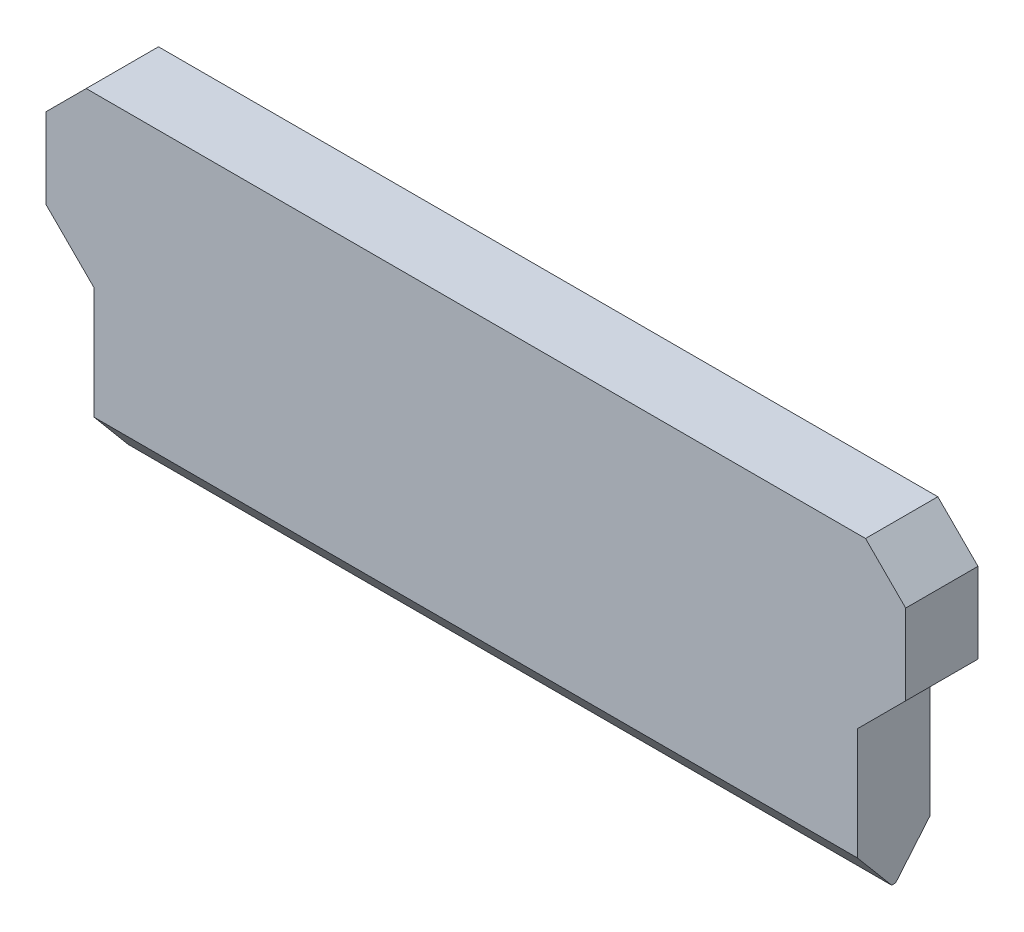
SolidWorks part; units mm, degrees
material "普通碳钢"
ref_plane "Front Plane" through (0, 0, 0) normal (0, 0, 1) x (1, 0, 0)
ref_plane "Top Plane" through (0, 0, 0) normal (0, 1, 0) x (1, 0, 0)
ref_plane "Right Plane" through (0, 0, 0) normal (1, 0, 0) x (0, 0, -1)
sketch "Sketch1" plane through (0, 0, 0) normal (0, 0, 1) x (1, 0, 0)
  line L0 (-194, 80) -> (194, 80)
  line L1 (194, 80) -> (214, 60)
  line L2 (214, 60) -> (214, 20)
  line L3 (214, 20) -> (190, -4)
  line L4 (190, -4) -> (190, -80)
  line L5 (190, -80) -> (-190, -80)
  line L6 (0, 129.5984) -> (0, -154.525) construction
  line L7 (-190, -4) -> (-190, -80)
  line L8 (-214, 20) -> (-190, -4)
  line L9 (-214, 60) -> (-214, 20)
  line L10 (-194, 80) -> (-214, 60)
  point P11 (0, -80)
  point P15 (0, 80)
  dimension "D1" = 214
  dimension "D3" = 40
  dimension "D4" = 20
  dimension "D5" = 45
  dimension "D6" = 45
  dimension "D7" = 160
  dimension "D8" = 190
  dimension "D9" = 80
extrude "Boss-Extrude1" add sketch "Sketch1" along normal mid plane 36
sketch "Sketch2" plane through (0, 0, 0) normal (1, 0, 0) x (0, 0, -1)
  line L1 (-18, -80) -> (18, -80) construction
  line L2 (-1, -80) -> (-18, -59.7402)
  line L3 (-18, -80) -> (-18, -4) construction
  line L4 (1, -80) -> (18, -59.7402)
  line L5 (18, -80) -> (18, -4) construction
  line L6 (-18, -59.7402) -> (-18, -80)
  line L7 (-18, -80) -> (-1, -80)
  line L8 (1, -80) -> (18, -80)
  line L9 (18, -80) -> (18, -59.7402)
  dimension "D1" = 2
  dimension "D2" = 1
  dimension "D3" = 50
  dimension "D4" = 50
extrude "Cut-Extrude1" cut sketch "Sketch2" against normal mid plane 428
